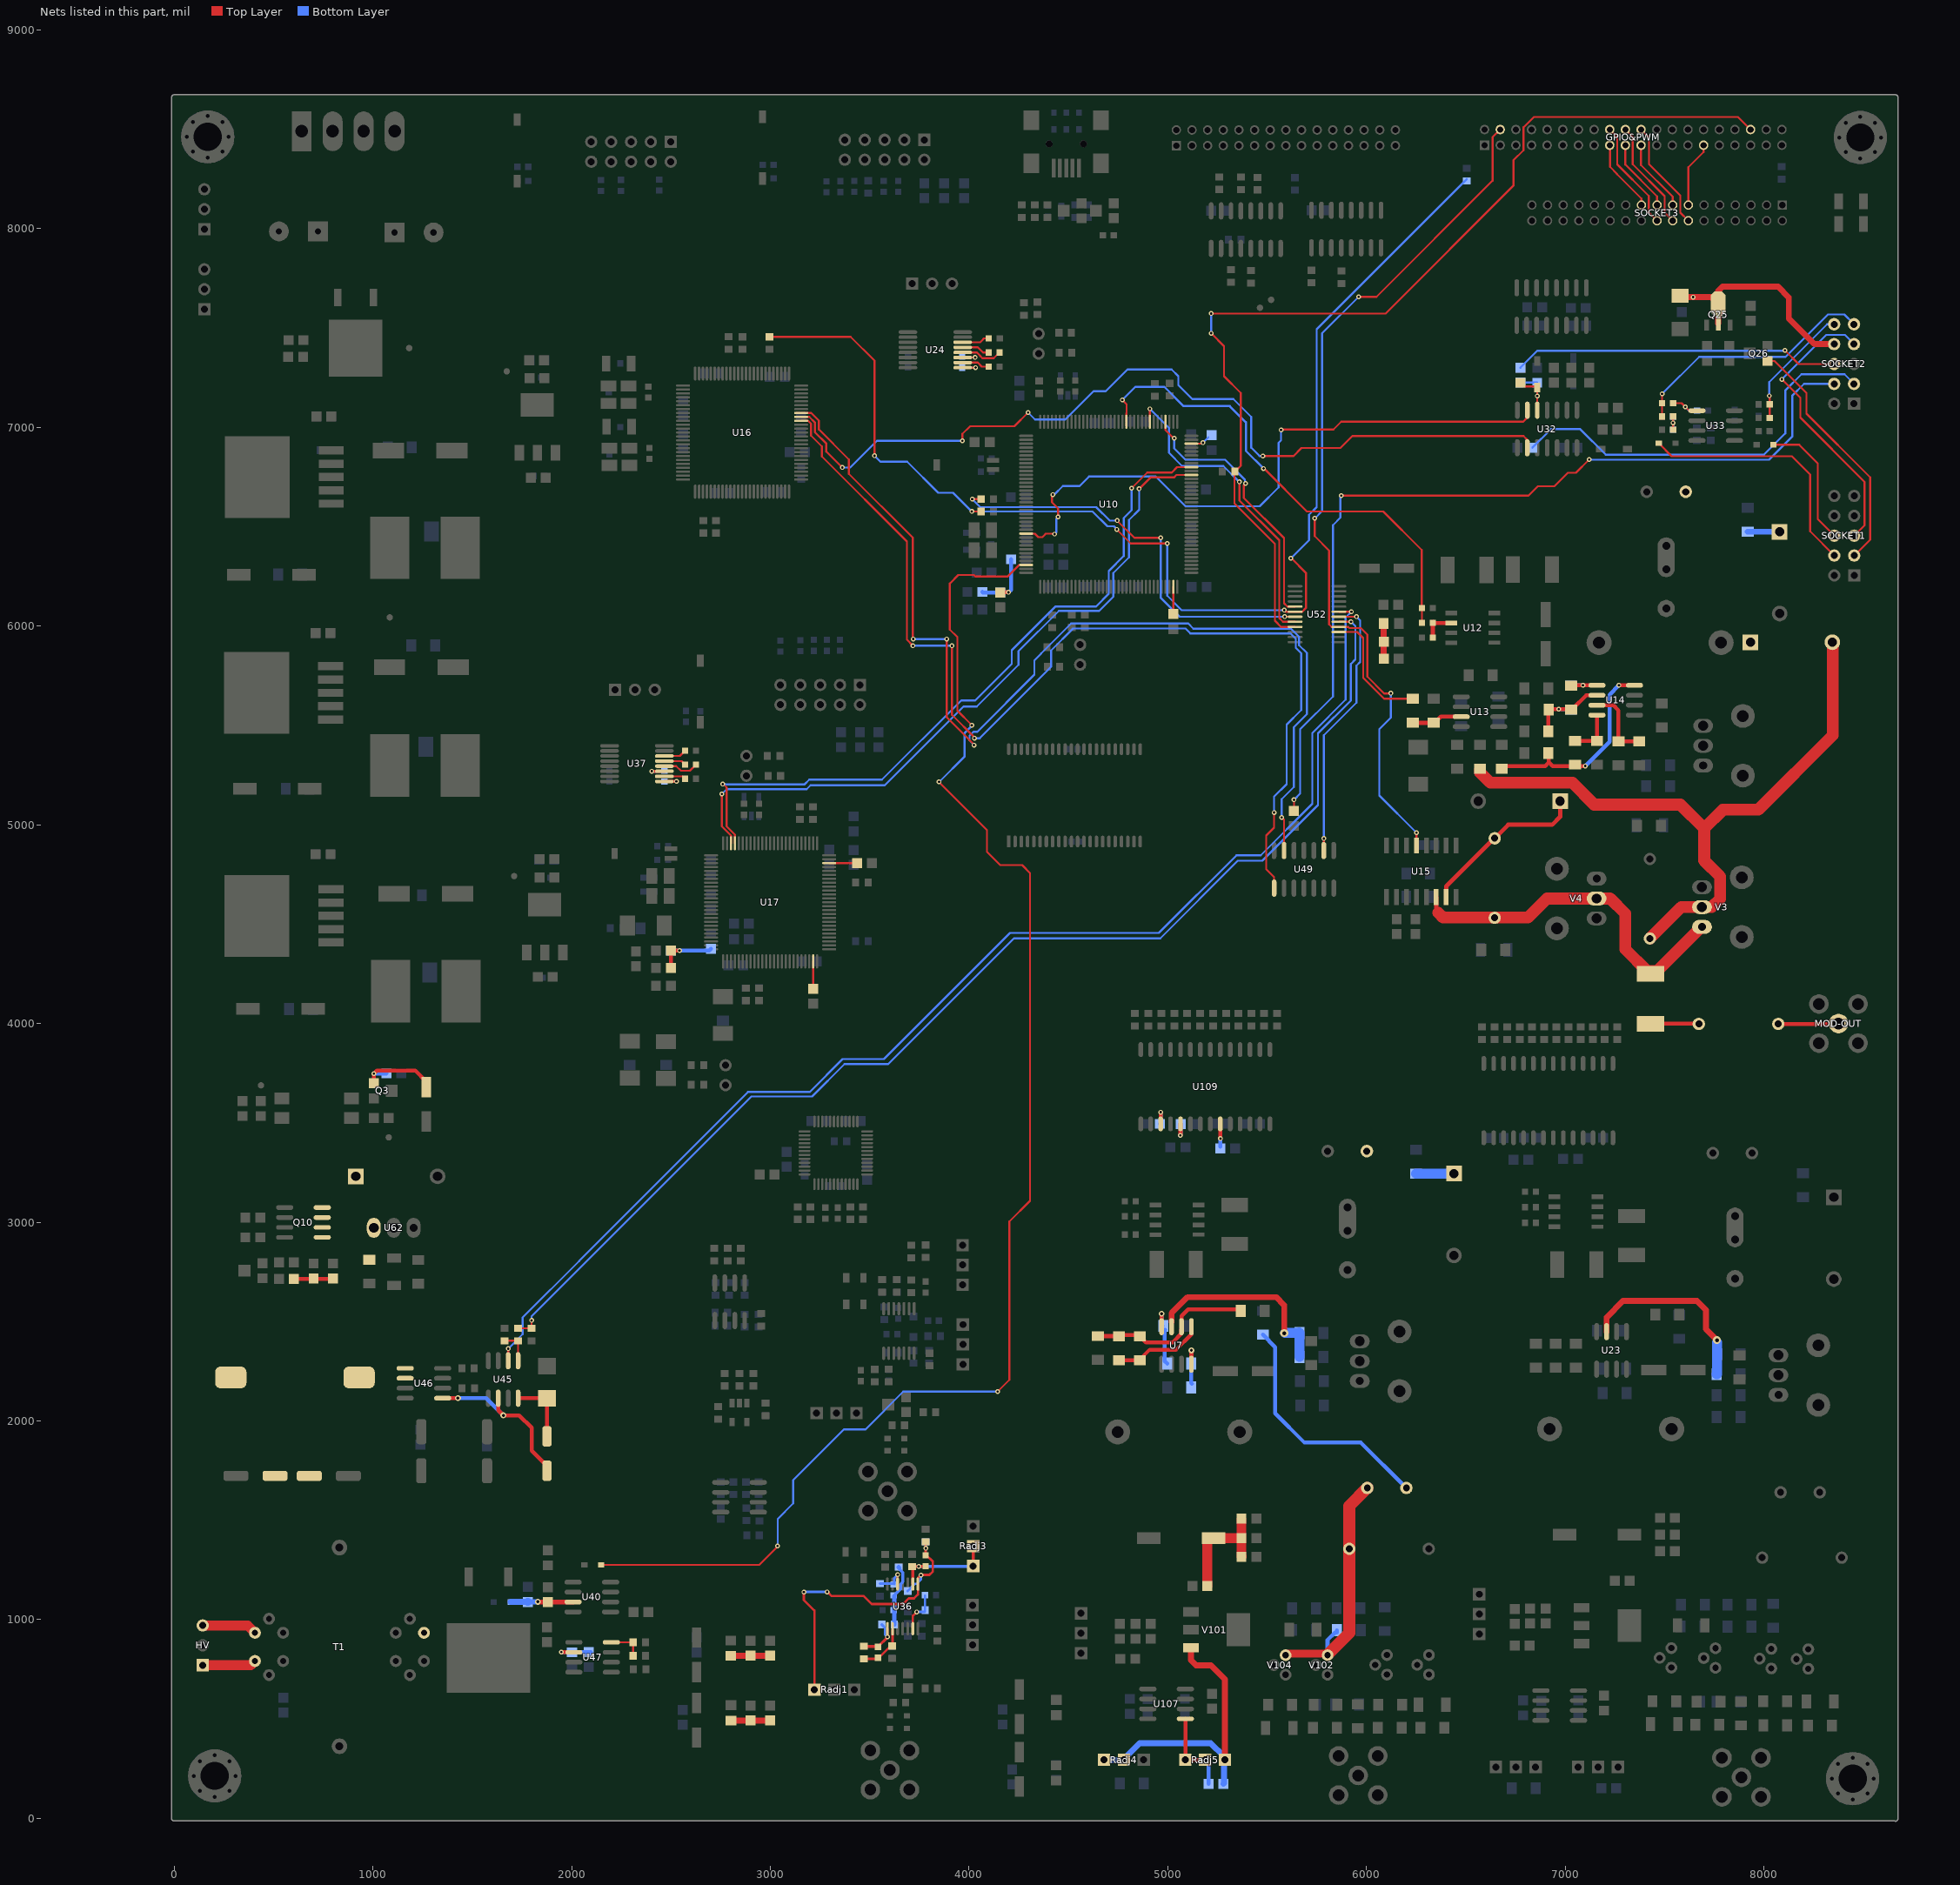
[diagram p0: the nets of this part, all layers, seen from the top]
# Altium PCB MISC82309.PcbDoc (part 9 of 14)
Units mil, origin at the board's own origin, x right, y up, seen from the top; angles counter-clockwise.
Board outline 8687.03 x 8687.86 mil, 4 copper layers (Top Layer, GND, POWER, Bottom Layer); 747 components, 583 nets, 2530 pads, 1834 vias.

## Via types
v1: diameter 24, hole 12, Top Layer to Bottom Layer, 1799 vias
v2: diameter 30, hole 15, Top Layer to Bottom Layer, 26 vias
v3: diameter 40, hole 20, Top Layer to Bottom Layer, 9 vias

## Nets (pads, with @x,y where several pads share a name; then routed paths per layer and width w, separated by ;. In a path a pad name is that pad's centre, name@x,y a point inside that pad or via, vN(x,y) a via of type N, cw(c..) or ccw(c..) an arc to the next point about the centre after c; other vN are vias at no path point) (continued)
HV-CLK: R347.2 R358.2 R391.2 U52.18 | length 6308.5
  Top Layer w10: R347.2@2996,7455.5 3404.5,7455.5 3524,7336 v1(3524,6857) ; v1(4014,6577) R391.2@4060.5,6577 ; v1(4744,6487) 4744,6486 4814,6416 v1(4997,6416) ; v1@5593.2,6072.8 U52.18@5640.76,6072.8 5676.8,6072.8 5695,6091 5695,6254 5695,6261 5695,6268 v1@5623,6340 ; v1@5619,6340 v1(5619,6342)
  Bottom Layer w10: v1(3524,6857) 3554,6827 3689,6827 3845,6671 3920,6671 v1(4014,6577) 4621,6577 4696,6502 4729,6502 v1(4744,6487) v1@4744,6486 ; v1(4997,6416) 4997,6153 5070,6080 v1(5586,6080) ; v1@5619,6340 v1(5619,6342) ; v1@5620,6342 5710.5,6432.5 5710.5,6560.5 5749,6599 5749,7494 R358.2@6504.5,8249.5
HV-CONTROL: U10.112 U52.17 | length 1331.3
  Top Layer w10: U10.112@4988.43,7028.35 4988.43,6986.57 5029,6946 v1(5032,6946) ; 5383,6709 5383,6645 5585,6443 5585,6115 5601.61,6098.39 U52.17@5640.76,6098.39
  Bottom Layer w10: v1(5032,6946) 5032,6894 5089,6837 5288,6837 5388,6737 5388,6731.06 5389,6730.06 v1@5389,6723 ; v1@5390,6719 v1(5391,6718)
HV-SHUTDOWN: U45.2 U52.7 | length 6403.5
  Top Layer w10: U45.2@1681,2303.49 v1(1681,2364) ; U52.7@5861.24,6072.8 v1(5924.2,6072.8)
  Bottom Layer w10: v1(1681,2364) 1754,2437 1754,2521 2038,2805 2038,2806 2888,3656 3199,3656 3364,3821 3571,3821 4206,4456 4955,4456 5346,4847 5468,4847 5727,5106 5727,5462 5895,5630 5895,6043.59 v1(5924.2,6072.8)
HV_CLK: U49.9 U52.6 | length 1352.7
  Top Layer w10: U49.9@5785,4870.49 v1(5785,4931) v1@5785,4937 ; U52.6@5861.24,6047.2 v1(5949.2,6047.2)
  Bottom Layer w10: v1(5785,4931) 5785,5451 5949.2,5615.2 5949.2,5801 5968,5819.8 5968,6029 v1@5953,6044 ; v1@5949.2,6044 v1(5949.2,6047.2)
HV_OUT+: HV.1 T1.7 | length 271.6
  Top Layer w50: HV.1@144,771 385.67,771 T1.7@406.8,792.13
HV_OUT-: HV.3 T1.8 | length 278.2
  Top Layer w50: HV.3@144,971 369.67,971 T1.8@406.8,933.87
HV_PWM: R285.1 R286.2 U52.5 | length 6220.6
  Top Layer w10: R285.1@1731,2466.5 R286.2@1799,2466.5 v1(1799,2506) ; U52.5@5861.24,6021.61 v1(5921.61,6021.61)
  Bottom Layer w10: v1(1799,2506) 1799,2527 2905,3633 3210,3633 3373,3796 3593,3796 4226,4429 4962,4429 5352,4819 5476,4819 5756,5099 5756,5460 5921.61,5625.61 5921.61,5810 5944.16,5832.54 5944.16,5999.84 v1@5923,6021 ; v1@5921.61,6021 v1(5921.61,6021.61)
HV_S: U10.26 U32.6 | length 3227.8
  Top Layer w10: U10.26@4287.65,6465.36 4330.7,6465.36 4348.06,6448 4369.06,6448 4379.03,6457.97 ; 4379,6458 4386,6465 4428,6465 v1(4430,6463) ; v1@4417,6657 4417,6623 4448,6592 v1(4448,6549) ; v1@5572,6989 5833,6989 5873,7029 6789,7029 6809,7049 U32.6@6809,7086.49
  Bottom Layer w10: v1(4422,6662) 4429,6662 4472,6705 4556,6705 4604,6753 4939,6753 5089,6603 5463,6603 5558,6698 5558,6769 ; 4439,6472 4439,6540 ; 5558,6775 5558,6769 ; 5558,6906 5558,6899 ; v1(5570,6987) 5570,6935 5558,6923 5558,6899 ; 5558,6769 5558,6899
HV_SENSOR: D33.2 U10.34 | length 7432.9
  Top Layer w10: D33.2@2149.32,1276 2944,1276 3038,1370 3037,1370 v1(3036,1371) ; v1@3848.5,5215.5 4090,4974 4090,4864 4157,4797 4267,4797 4307,4757 4307,3108 4203,3004 4203,2207 v1(4144,2148) ; v1@4012,5503 3941,5574 3941,5945 3903,5983 3903,6214 3946,6257 4025,6257 4033,6249 4193.6,6249 4252.48,6307.88 U10.34@4287.65,6307.88
  Bottom Layer w10: v1@3037,1370 3037,1507 3115,1585 3115,1703 3370,1958 3479,1958 3669,2148 v1(4144,2148) ; v1@3850,5217 3978,5345 3978,5463 v1@4013,5498
  other v1: 3849,5216 4014,5501
HV_SET: R392.2 U52.19 | length 2093.4
  Top Layer w10: v1(4016.17,6639.17) R392.2@4060.5,6639.17 ; v1(4746,6531) 4746,6530 4832,6444 v1(4964,6444) ; v1(5587.8,6047.2) U52.19@5640.76,6047.2
  Bottom Layer w10: v1(4016.17,6639.17) 4056.35,6599 4640,6599 4708,6531 v1@4744,6531 ; v1@4745,6530 v1@4744,6531 ; v1@4746,6530 v1(4746,6531) v1@4744,6531 ; v1(4964,6444) 4964,6143 5059.8,6047.2 v1(5587.8,6047.2)
HV_SINGLE: R166.1 SOCKET2.6 | length 1643.8
  Top Layer w10: v1(8105,7388) 8174,7319 SOCKET2.6@8353,7319
  Bottom Layer w10: R166.1@6774,7300.5 6859.05,7385.55 8077.45,7385.55 8102.55,7385.55 v1(8105,7388)
HV_VCC: C227.2 C228.2 L13.2 T1.2
INK-LED_A: R212.2 SOCKET2.3 | length 2023.2
  Bottom Layer w10: R212.2@6834.5,6898 6927.5,6991 7076,6991 7204,6863 8000,6863 8107,6970 8107,7185 8189,7267 8405,7267 SOCKET2.3@8453,7219
INK-LED_B: R386.2 SOCKET2.4 | length 4523.9
  Top Layer w10: R386.2@5635,5066 R386.2@5635,5069.5 v1(5635,5126) ; v1(5873,6657) 6815,6657 6862,6704 6945,6704 7013,6772 7054,6772 v1(7120,6838)
  Bottom Layer w10: v1(5635,5126) 5666,5157 5666,5481 5831,5646 5831,6508 5869,6546 5869,6653 v1(5873,6657) ; v1(7120,6838) 7121,6837 8026,6837 8142,6953 8142,7159 8202,7219 SOCKET2.4@8353,7219
INK_DETECTING: U10.98 U17.98 | length 3576.2
  Top Layer w10: v1@2757,5157 2756,5156 v1(2756,5155) 2756,4992 2802.15,4945.85 U17.98@2802.15,4907.24 ; v1(4856,6691) 4913,6748 5031,6748 5043.64,6760.64 U10.98@5118.35,6760.64
  Bottom Layer w10: v1@2758,5157 2780,5179 3183,5179 3203,5199 3576,5199 3972,5595 4039,5595 4249,5805 4249,5874 4452,6077 4655,6077 4726,6148 4726,6267 4805,6346 4805,6534 4856,6585 v1(4856,6691)
INK_FLOW_A: D31.2 SOCKET1.4 | length 1284.9
  Top Layer w10: D31.2@7470.68,6920 7535.68,6855 8140,6855 8232,6763 8232,6477 SOCKET1.4@8354,6355
INK_FLOW_B: D131.2 SOCKET1.6 | length 661
  Top Layer w10: D131.2@8047.32,6913 8177,6913 8271,6819 8271,6538 SOCKET1.6@8354,6455
INK_FLOW_SA: R172.2 R173.2 SOCKET2.9 | length 1264.8
  Top Layer w10: R173.2@7487.5,7055 R172.2@7487.5,7122 v1(7487.5,7168.5)
  Bottom Layer w10: v1(7487.5,7168.5) 7674,7355 8109,7355 8322,7568 8404,7568 SOCKET2.9@8453,7519
INK_FLOW_SB: R372.2 R373.2 SOCKET2.10 | length 625
  Top Layer w10: R373.2@8028.5,7048 R372.2@8028.5,7116 v1@8028.5,7157.5
  Bottom Layer w10: v1(8027,7159) 8027,7228 8318,7519 SOCKET2.10@8353,7519
INK_PRINTING: U10.100 U17.97 | length 3629.5
  Top Layer w10: v1@2762,5206 2780,5188 2780,4992.04 2821.83,4950.21 U17.97@2821.83,4907.24 ; v1(4818,6694) 4897.02,6773.02 5020.02,6773.02 5047,6800 U10.100@5118.35,6800.01
  Bottom Layer w10: v1@2765,5205 2766,5204 3173,5204 3196,5227 3562,5227 3961,5626 4031,5626 4215,5810 4215,5879 4434,6098 4638,6098 4703,6163 4703,6277 4779,6353 4779,6544 4818,6583 4818,6603 ; 4818,6596 4818,6603 ; v1(4818,6694) 4818,6603
  other v1: 2761,5205
INPUT0: GPIO&PWM.18 SOCKET3.18 | length 557.2
  Top Layer w10: GPIO&PWM.18@7223.92,8498.74 7254.83,8467.83 ; 7255,8468 7262,8461 7262,8323 7420,8165 7420,8082.34 SOCKET3.18@7462.08,8040.26
INPUT1: GPIO&PWM.19 SOCKET3.17 | length 367
  Top Layer w10: GPIO&PWM.19@7302.66,8420 7302.66,8322.34 7462.08,8162.92 SOCKET3.17@7462.08,8119
INPUT3: GPIO&PWM.17 SOCKET3.19 | length 371.6
  Top Layer w10: GPIO&PWM.17@7225,8425 7225,8311 7261,8275 7261,8274 7383.34,8151.66 SOCKET3.19@7383.34,8119
INPUT4: GPIO&PWM.21 SOCKET3.15 | length 367
  Top Layer w10: GPIO&PWM.21@7381.4,8420 7381.4,8320.6 7540.82,8161.18 SOCKET3.15@7540.82,8119
INPUT5: GPIO&PWM.20 SOCKET3.16 | length 557.1
  Top Layer w10: GPIO&PWM.20@7302.66,8498.74 7339,8462.4 7339,8325 7500,8164 7500,8081.08 SOCKET3.16@7540.82,8040.26
INPUT6: GPIO&PWM.29 SOCKET3.13 | length 332.8
  Top Layer w10: SOCKET3.13@7619.56,8119 7619.56,8309 7696.36,8385.8 GPIO&PWM.29@7696.36,8420
INPUT7: GPIO&PWM.22 SOCKET3.14 | length 557.1
  Top Layer w10: GPIO&PWM.22@7381.4,8498.74 7421,8459.14 7421,8325 7579,8167 7579,8080.82 SOCKET3.14@7619.56,8040.26
LASER_CTRL: Q26.1 SOCKET1.3 | length 1246.4
  Top Layer w10: Q26.1@8018,7334 8053,7334 8151,7236 8214,7173 8214,7069 8534,6749 8534,6435 SOCKET1.3@8454,6355
LASER_DRV: C221.2 D40.2 Q25.2 SOCKET2.8 | length 1205.2
  Top Layer w30: D40.2@7578,7662.86 7584.86,7656 7735.43,7656 Q25.2@7770,7621.43 ; Q25.2@7770,7523.01 Q25.2@7770,7621.43 ; SOCKET2.8@8353,7419 8254,7419 8125,7548 8125,7654 8071,7708 7791,7708 7770,7687 Q25.2@7770,7621.43
  Bottom Layer w30: C221.2@7585,7655.5 v1(7643.5,7655.5)
MCH_DRV: SOCKET1.5 SOCKET2.7 | length 1455.3
  Top Layer w10: v1(8090,7242) 8183,7149 8183,7049 8506,6726 8506,6507 SOCKET1.5@8454,6455
  Bottom Layer w10: v1(8090,7242) 8124.5,7276.5 8313,7465 8407,7465 SOCKET2.7@8453,7419
MOD-CLK: U16.66 U49.1 | length 5363.3
  Top Layer w10: U16.66@3155.24,7033.06 3190.41,7033.06 3205,7018.46 3205,6959 3259.83,6904.17 3259.83,6853.17 3687,6426 3687,5932 v1(3718,5901) ; v1(3914,5901) 3914,5554 4029,5439 v1@4029,5438 ; 5534,4738 5495,4777 5495,4946 5535,4986 v1(5535,5062) ; U49.1@5535,4681.51 5535,4738
  Bottom Layer w10: v1(3718,5901) v1(3914,5901) ; v1(4027,5436) 4054,5436 4413,5795 4413,5877 4524,5988 5089,5988 5114,5963 5618,5963 5644,5937 5644,5891 5671.5,5863.5 5671.5,5577.5 5598,5504 5598,5205 5535,5142 v1(5535,5062)
MOD-CONTROL: U10.116 U52.20 | length 1597.8
  Top Layer w10: U10.116@4909.69,7028.35 v1(4909.69,7093.31) ; v1@5361,6727 5361,6632 5561,6432 5561,6040.06 5579.44,6021.61 U52.20@5640.76,6021.61
  Bottom Layer w10: v1(4909.69,7093.31) 5006,6997 5006,6872 5072,6806 5280,6806 v1(5360,6726)
MOD-LED_A: U16.67 U32.9 | length 4451.5
  Top Layer w10: U16.67@3155.24,7052.74 3196.26,7052.74 3224,7025 3224,6976 3282,6918 3282,6878 v1(3362,6798) ; v1(3967,6933) 3967,6967 4006,7006 4228,7006 v1(4297,7075) ; v1(5478,6856) 5633,6856 5673,6896 5868,6896 5929,6957 6790,6957 6809,6938 U32.9@6809,6897.51
  Bottom Layer w10: v1(3362,6798) 3402,6798 3537,6933 v1(3967,6933) ; v1(4297,7075) 4332,7040 4484,7040 4626,7182 4688,7182 4797,7291 5019,7291 5053,7257 5053,7213 5123,7143 5330,7143 5420,7053 5420,6898 5462,6856 v1(5478,6856)
MOD-LED_B: U16.68 U49.13 | length 5310.6
  Top Layer w10: U16.68@3155.24,7072.43 3205.57,7072.43 3244.07,7033.93 3244.07,6989.93 3395.47,6838.53 3395.47,6766.53 3717,6445 v1@3717,5937 ; v1(3888,5935) 3888,5542 4003,5427 ; 4003,5426.06 4017.06,5412 ; v1(5573,5037) 5585,5025 U49.13@5585,4870.49
  Bottom Layer w10: v1(3719,5935) v1(3888,5935) ; v1@4024,5403 4003,5424 4003,5449 4022.5,5468.5 4041.5,5468.5 4329,5756 4329,5827 4363,5861 ; v1(4025,5401) v1@4025,5405 ; 4363,5862 4514,6013 5103,6013 5129,5987 5620,5987 5661,5946 5661,5904 5700,5865 5700,5557 5634,5491 5634,5190 5573,5129 v1(5573,5037)
MOD-PWM: R72.2 U52.3 | length 626.9
  Top Layer w10: U52.3@5861.24,5970.43 5952.57,5970.43 5983,5940 5983,5740 6088,5635 R72.2@6232,5635
MOD-SET: GPIO&PWM.36 R508.2 U52.21 | length 5112
  Top Layer w10: v1(5218,7474) 5283,7409 5283,7257 5367,7173 5367,6807 5336,6776 5336,6617 5539,6414 5539,6027 5569.98,5996.02 U52.21@5640.76,5996.02 ; v1(5218,7573) 6096,7573 6739,8216 6739,8344 6790,8395 6790,8510 6842,8562 7869.32,8562 GPIO&PWM.36@7932.58,8498.74
  Bottom Layer w10: v1(5218,7474) v1(5218,7573)
MOD-SHUTDOWN: GPIO&PWM.4 U15.13 U52.4 | length 4403.1
  Top Layer w10: v1@5738,6543 v1(5739,6543) ; v1@5739,6542 5739,6453 5811.83,6380.17 5811.83,6009.17 U52.4@5824.98,5996.02 ; U52.4@5829.02,5996.02 U52.4@5861.24,5996.02 5907.98,5996.02 5914,5990 5971,5990 6004,5957 6004,5746 6089,5661 6123,5661 v1(6122,5662) ; v1(5960,7657) 6050,7657 6634,8241 6634,8460 GPIO&PWM.4@6672.74,8498.74 ; U15.13@6251,4896 v1(6251,4960)
  Bottom Layer w10: v1@5738,6541 5739,6541 5776,6578 5776,7473 v1(5960,7657) ; v1@6122,5659 6122,5539 6064,5481 6064,5147 v1(6251,4960)
MOD_CTRL: R67.2 R68.2 U10.122 | length 2439.6
  Top Layer w10: v1(4771,7138) 4793,7116 4793,7073 4791.58,7071.58 U10.122@4791.58,7028.35 ; v1(5482,6793) 5484,6793 5700,6577 6084,6577 6278,6383 R68.2@6278,6095 ; R67.2@6278.5,6016 R68.2@6278.5,6089.5
  Bottom Layer w10: v1(4771,7138) 4837,7204 4983,7204 5080,7107 5312,7107 5393,7026 5393,6882 v1(5482,6793)
MOD_OUT: C62.2 MOD-OUT.1 | length 286.8
  Top Layer w20: C62.2@8072,3998 8356,3998 MOD-OUT.1@8358,3996
NetC17_2: C17.2 Q3.1 R15.1 | length 427.9
  Top Layer w20: Q3.1@1005,3699 v1(1005,3748) ; v1@1007,3749 1021,3763 1214,3763 1268,3709 C17.2@1268,3692 ; C17.2@1269,3680.23 C17.2@1269,3692
  Bottom Layer w20: v1@1008,3748 1067.5,3748 R15.1@1068.5,3749
NetC23_1: C23.1 R17.2 R18.1 R38.2 U7.2 | length 851.8
  Top Layer w15: R38.2@4848,2427 R38.2@4852,2423 ; R38.2@4860,2426 R38.2@4860,2432
  Top Layer w20: R17.2@4648,2427 4751,2427 4756,2432 4860,2432 R38.2@4861,2431 ; R38.2@4860,2426 4890,2396 5025,2396 5068,2439 U7.2@5068,2461 ; U7.2@5069,2474.49 5069,2529 5102,2562 5361,2562 R18.1@5364,2559
NetC23_2: C23.2 R38.1 U7.1 | length 450.3
  Top Layer w20: C23.2@4755,2306 4856,2306 4909,2359 5042,2359 5120,2437 U7.1@5120,2468
NetC24_1: C24.1 R26.1 U7.8 | length 256.1
  Top Layer w20: U7.8@5119,2268 U7.8@5119,2285.51 v2(5119,2355)
  Bottom Layer w20: v2@5118,2355 5117,2354 R26.1@5117,2289 5117,2192 C24.1@5121,2188
NetC25_1: C25.1 R26.2 U7.4 | length 303.6
  Top Layer w20: U7.4@4969,2474.49 v2(4969,2540)
  Bottom Layer w20: v2(4969,2540) 4969,2483 C25.1@4973,2479 ; C25.1@4986,2459 4985,2458 4985,2301 R26.2@4997,2289
NetC27_1: C27.1 R25.1 U7.3 | length 1025.5
  Top Layer w20: U7.3@5019,2474.49 U7.3@5019,2499
  Top Layer w30: U7.3@5019,2499 5019,2542 5100,2623 5545,2623 5586,2582 v3(5586,2442)
  Bottom Layer w20: v3@5586,2443 5587,2442 v3@5591,2442
  Bottom Layer w50: v3@5591,2444 5658,2444 5660,2446 5663,2443 C27.1@5663,2442 R25.1@5663,2322
NetC29_1: C29.1 D5.2 L111.1 R19.2 R39.2 | length 1413.4
  Bottom Layer w20: R19.2@5479,2434 5541,2372 5541,2038 5688,1891 5972,1891 L111.1@6192,1671
  Bottom Layer w50: R39.2@6249,3245 6432,3245 D5.2@6436,3241
NetC30_2: C30.2 U109.19 | length 117.4
  Top Layer w20: v1(5063,3437) 5064,3438 U109.19@5064,3494.99
  Bottom Layer w20: v1@5062,3436 v1(5063,3437) 5064.5,3438.5 C30.2@5064.5,3494
NetC32_1: C32.1 U109.17 | length 119.5
  Top Layer w20: U109.17@4964,3494.99 v1(4964,3554)
  Bottom Layer w20: C32.1@4960.5,3495 4964,3498.49 v1(4964,3554)
NetC33_2: C33.2 U109.23 | length 115.8
  Top Layer w20: U109.23@5264,3494.99 5264,3422 v1(5265,3421)
  Bottom Layer w20: C33.2@5264,3380 5265,3381 v1(5265,3421)
NetC35_2: C35.2 C36.2 L11.2 R276.1 | length 326.3
  Top Layer w20: C36.2@4157,6168.5 4158.51,6170 v1(4199,6170)
  Bottom Layer w20: L11.2@4066.5,6172 4070,6168.5 C35.2@4143,6168.5 ; C35.2@4157,6168.5 4158.5,6170 v1@4198,6170 ; v1@4204,6175 4211.5,6182.5 R276.1@4211.5,6336
NetC42_2: C42.2 R67.1 U12.2 | length 174.1
  Top Layer w20: R67.1@6331,6013.5 R67.1@6333.5,6016 C42.2@6333.5,5940.5 ; R67.1@6334,6021 6339,6016 U12.2@6427,6016
NetC45_1: C45.1 R72.1 U13.3 | length 255.4
  Top Layer w20: R72.1@6234,5513 6343,5513 6374,5544 U13.3@6476.51,5544
NetC47_1: C47.1 R77.2 U14.1 | length 165.9
  Top Layer w20: C47.1@7043,5702 v1(7089,5702) 7091,5702 U14.1@7159.51,5702
  Bottom Layer w20: R77.2@7040,5703 7041,5702 v1(7089,5702)
NetC47_2: C47.2 R76.2 R77.1 R78.2 U14.2 | length 431.3
  Top Layer w20: R76.2@6915,5470 6915,5580 6917,5582 v1(6967,5582) 7028,5582 C47.2@7030,5580 ; C47.2@7035,5584 7038,5584 7106,5652 U14.2@7159.51,5652
  Bottom Layer w20: v1(6967,5582) R77.1@7019,5582
NetC48_1: C48.1 R75.2 U14.4 | length 234.8
  Top Layer w20: R75.2@7049,5423 7158,5423 7160,5425 U14.4@7160,5548
NetC49_1: C49.1 R73.1 R75.1 U14.8 | length 1037.3
  Top Layer w20: R73.1@6681,5283 6694,5296 6899,5296 6916,5313 6916,5358 C49.1@6915,5359 ; 6916,5317 6937,5296 7036,5296 7037,5297 R75.1@7045,5297 ; R75.1@7049,5303 7056,5296 v1(7101,5296) ; v1@7274,5702 U14.8@7348.49,5702
  Bottom Layer w20: v1(7101,5296) 7223,5418 7223,5655 v1(7270,5702)
NetC51_1: C51.1 R82.1 U14.3 | length 367.2
  Top Layer w20: U14.3@7166,5601 7243,5601 7268,5576 C51.1@7268,5420 R82.1@7364,5420 ; R82.1@7370,5422 R82.1@7372,5420
NetC54_1: C54.1 D11.2 D13.2 R74.2 | length 142
  Bottom Layer w30: R74.2@7918,6475 D13.2@8060,6475
NetC55_2: C55.2 D11.1 R71.1 V3.2 | length 3387.1
  Top Layer w60: R71.1@6571,5262 R71.1@6571,5276 ; R71.1@6571,5277 R71.1@6571,5276 ; C55.2@7427,4429 7584,4586 V3.2@7688,4586 7737,4586 7779,4628 7779,4740 7699,4820 7699,4982 ; D11.1@8347,5903 8346,5902 8346,5451 7971,5076 7793,5076 7699,4982 ; R71.1@6571,5276 6571,5264 6623,5212 7036,5212 7146,5102 7579,5102 7699,4982
NetC58_1: C58.1 R89.1 U15.6 V3.3 V4.2 | length 1801.7
  Top Layer w20: U15.6@6351,4636 6351,4582 6368,4565
  Top Layer w60: 6361,4558 6386,4533 6812,4533 6908,4629 V4.2@7158,4629 7226,4629 7302,4553 7302,4374 7412,4264 7462,4264 7683,4485 V3.3@7687,4485
NetC58_2: C58.2 D15.2 U15.7 | length 837.6
  Top Layer w22: U15.7@6401,4636 6401,4690 C58.2@6636,4925 ; C58.2@6634.5,4926.5 C58.2@6637,4929 ; C58.2@6645,4932 6713,5000 6934,5000 6974,5040 D15.2@6974,5114
NetC62_1: C62.1 R89.2 | length 235.4
  Top Layer w20: R89.2@7430,3999.02 C62.1@7663.98,3999.02
  Top Layer w30: C62.1@7663.98,3999.02 C62.1@7665,3998
NetC66_2: C66.2 FB3.2 R91.1 | length 175.9
  Top Layer w30: FB3.2@6082,6010 6086.5,6005.5 C66.2@6086.5,5921 6086.5,5920.5 R91.1@6086.5,5836
NetC70_2: C70.2 C71.2 L14.2 R225.1 | length 336.9
  Top Layer w20: L14.2@2499.5,4280 C70.2@2499.5,4367 v1(2542.99,4366.99)
  Bottom Layer w20: C71.2@2499.5,4367 2559,4367 2692.5,4367 R225.1@2702,4376.5
NetC78_1: C78.1 D10.2 Q10.5 Q10.6 Q10.7 Q10.8 U62.1
NetC91_1: C91.1 U24.3 | length 129.8
  Top Layer w10: U24.3@3967.8,7351.61 4030.61,7351.61 v1(4031,7352)
  Bottom Layer w10: C91.1@3966,7355.5 3969.5,7352 v1(4031,7352)
NetC91_2: C91.2 U24.1 | length 132.6
  Top Layer w10: U24.1@3967.8,7300.43 4032.43,7300.43 v1(4033,7301)
  Bottom Layer w10: C91.2@3966,7300.5 4032.5,7300.5 v1(4033,7301)
NetC92_1: C92.1 U24.5 | length 141.4
  Top Layer w10: U24.5@3967.8,7402.8 4044.2,7402.8 4070,7377 C92.1@4098.5,7377
NetC92_2: C92.2 U24.4 | length 211
  Top Layer w10: U24.4@3967.8,7377.2 4039.74,7377.2 4055,7361.94 4055,7360 4067,7348 4124.5,7348 C92.2@4153.5,7377
NetC93_2: C93.2 U24.2 | length 139
  Top Layer w10: U24.2@3967.8,7326.02 4043.98,7326.02 4064,7306 C93.2@4098.5,7306
NetC94_2: C94.2 U24.6 | length 140.4
  Top Layer w10: U24.6@3967.8,7428.39 4056.33,7428.39 4072,7444.06 4072,7445 4075,7448 C94.2@4099.5,7448
NetC157_1: C157.1 R44.2 R45.2 R46.1 TC2.2 | length 564.2
  Top Layer w50: R44.2@5199.5,1170 5199.5,1400.5 TC2.2@5205,1406 ; TC2.2@5230.77,1411 R46.1@5370,1411 ; R45.2@5370.5,1505.5 R46.1@5370.5,1411 5370.5,1319.5 C157.1@5371,1319
NetC162_2: C162.2 D24.2 R166.2 R168.2 U32.5 | length 360.6
  Top Layer w10: C162.2@6774,7224.5 6792.5,7206 6853.07,7206 D24.2@6859,7200.07 U32.5@6859,7086.49
  Bottom Layer w10: R166.2@6774,7225.5 6858,7225.5 R168.2@6859,7224.5 v1(6859,7158)
NetC163_1: C163.1 R173.1 R174.1 R175.2 | length 134.5
  Top Layer w10: R175.2@7542.5,6988 R173.1@7542.5,7055
  Bottom Layer w10: v1(7542,7023) v1@7542.5,7023 ; C163.1@7542.5,6988 v1@7542.5,7023 ; R174.1@7542.5,7055 v1@7542.5,7023
NetC164_2: C164.2 R172.1 U33.5 | length 203.1
  Top Layer w10: R172.1@7542.5,7122 7586,7122 7624,7084 U33.5@7662.51,7084
  Bottom Layer w10: v1(7604,7103) 7623,7084 C164.2@7663.5,7084
NetC166_1: C166.1 R187.2 R188.1 U36.1 | length 245.2
  Top Layer w14: R187.2@3480,865 3543,865 3589.23,911.23 U36.1@3589.23,954.8
  Bottom Layer w14: R188.1@3561.5,975 R188.1@3564.25,972.25 ; R188.1@3564,972 3578,958 3578,924 v1(3589,913)
NetC166_2: C166.2 R186.2 R187.1 U36.2 | length 248
  Top Layer w12: R187.1@3470,803.5 3541.5,803.5 3609,871 3610,871 3615,876 U36.2@3615,949
NetC167_1: C167.1 C168.2 R188.2 R189.1 | length 304.1
  Bottom Layer w15: C168.2@3630,1129 3655,1154 3655,1179 ; R189.1@3651,1262 3651,1253.48 3667.5,1236.98 3667.5,1225 3667.5,1215.02 3667.5,1190.5 3656,1179
  Bottom Layer w20: C168.2@3623,1120 3624,1119 3624,975.5 R188.2@3624.5,975 ; R189.1@3646,1262.01 R189.1@3646,1265.5
NetC168_1: C168.1 R192.2 U36.12 | length 167
  Top Layer w12: U36.12@3640.41,1179.2 3640.41,1225.41 v1(3641,1226)
  Bottom Layer w12: R192.2@3552,1181.5 3621.5,1181.5 3624,1179 3624,1209 v1@3636,1221
NetC169_1: C169.1 D27.1 R195.2 R196.2 Radj1.3 U36.8 | length 1614.2
  Top Layer w12: v1(3169,1139) 3169,1099 3222,1046 Radj1.3@3222,648 ; v1@3288,1140 3309,1119 3470,1119 3510,1079 3669,1079 3697,1107 3723,1107 3742.77,1126.77 U36.8@3742.77,1179.2 3742.77,1210.77 3757,1225 3800,1225 3818,1243 3818,1292 3782,1328 R196.2@3782,1392
  Bottom Layer w12: v1(3169,1139) 3170,1140 v1(3286,1140) ; D27.1@3691,1144 3728,1181 3738,1181 3758,1201 v1(3758,1224) ; R195.2@3782,1392.5 3782,1360 v1(3783,1359)
NetC169_2: C169.2 R194.2 Radj3.2 Radj3.3 U36.9 | length 495.2
  Top Layer w14: U36.9@3717.18,1179.2 R194.2@3717.18,1254.82 ; R194.2@3717.18,1261.82 3717,1262 3723,1268 v1(3747,1268) C169.2@3777,1268 ; Radj3.3@4021,1277 4021,1366 Radj3.2@4023,1368
  Bottom Layer w14: v1(3747,1268) 3846,1268 Radj3.3@4012,1268
NetC170_1: C170.1 R200.1 U36.6 | length 214.2
  Top Layer w12: U36.6@3717.18,954.8 3717.18,1019.18 v1(3737,1039)
  Bottom Layer w12: v1(3737,1039) 3776,1039 3778,1041 C170.1@3778,1121
NetC173_2: C173.2 FB19.2 R204.1 | length 198.4
  Top Layer w30: FB19.2@2802,492.61 R204.1@3000.39,492.61
NetC176_2: C176.2 FB20.2 R205.1 | length 189.4
  Top Layer w30: FB20.2@2801,818.61 R205.1@2990.39,818.61
NetC177_1: C177.1 U37.3 | length 124.8
  Top Layer w15: v1(2403.61,5269.61) U37.3@2466.8,5269.61
  Bottom Layer w15: v1(2403.61,5269.61) 2404.23,5269 C177.1@2465,5269
NetC177_2: C177.2 U37.1 | length 117.3
  Top Layer w15: U37.1@2466.8,5218.43 v1(2527.57,5218.43)
  Bottom Layer w15: C177.2@2467,5217.5 v1@2523.5,5217.5
NetC178_1: C178.1 U37.5 | length 112.1
  Top Layer w10: U37.5@2466.8,5320.8 2553.7,5320.8 C178.1@2571.5,5303
NetC178_2: C178.2 U37.4 | length 182.2
  Top Layer w10: U37.4@2466.8,5295.2 2526.8,5295.2 2550,5272 2595.5,5272 C178.2@2626.5,5303
NetC179_2: C179.2 U37.2 | length 109.7
  Top Layer w10: U37.2@2466.8,5244.02 2559.48,5244.02 C179.2@2571.5,5232
NetC180_2: C180.2 U37.6 | length 115.7
  Top Layer w10: U37.6@2466.8,5346.39 2544.89,5346.39 C180.2@2571.5,5373
NetC184_2: C184.2 D32.2 R216.2 U40.3 | length 316.1
  Top Layer w25: v2(1830,1090) 1831.5,1088.5 R216.2@1881,1088.5 1881.5,1089 U40.3@2007.51,1089
  Bottom Layer w20: v2@1829.5,1089.5 v2(1830,1090)
  Bottom Layer w25: C184.2@1780.5,1090 v2(1830,1090)
  Bottom Layer w30: D32.2@1693.32,1089 C184.2@1779.5,1089
  Bottom Layer w40: C184.2@1779.5,1089 C184.2@1780,1089.5 C184.2@1780.5,1090
NetC187_1: C187.1 Radj4.1 Radj4.2 Radj5.3 V101.3 | length 1466.6
  Top Layer w30: V101.3@5116,858.45 5116,796 5142,770 5218,770 5288,700 Radj5.3@5288,299
  Bottom Layer w30: Radj4.1@4694,294 4774,294 4859,379 5216,379 5283,312 5283,177.49 C187.1@5279.5,174
NetC187_2: C187.2 Radj5.1 Radj5.2 U107.1 | length 437.7
  Top Layer w20: Radj5.1@5088,295 Radj5.2@5188,295 5190,295 Radj5.2@5193,292 ; U107.1@5088.49,501 5088.49,305.51 Radj5.1@5089,305
  Bottom Layer w20: C187.2@5204.5,174 5204.5,308.5 Radj5.2@5205,309
NetC188_2: C188.2 L111.2 R153.2 V102.3 V104.3 | length 1281.2
  Top Layer w20: V102.3@5795.79,821.21 V102.3@5798,819
  Top Layer w40: V104.3@5593,821.21 5600.32,828.53 5805.47,828.53 5807.5,826.5 V102.3@5808,826
  Top Layer w50: V102.3@5807.5,826.5 V102.3@5808.5,827.5
  Top Layer w60: V102.3@5808,828 5913,933 C188.2@5913,1357 5913,1572.43 L111.2@6003.57,1663
  Bottom Layer w20: V102.3@5804,821.21 5804,898 R153.2@5842,936 ; R153.2@5851,936 R153.2@5851,947
NetC193_2: C193.2 R8.2 R12.1 | length 197.9
  Top Layer w20: R12.1@602.5,2714 795.5,2714 R8.2@799,2717.5
NetC214_1: C214.1 U10.106 | length 98.9
  Top Layer w10: U10.106@5118.35,6918.12 5172.12,6918.12 v1(5177,6923)
  Bottom Layer w10: v1(5177,6923) C214.1@5204,6950
NetC215_1: C215.1 U10.71 | length 137.2
  Top Layer w10: U10.71@5027.8,6197.65 5028,6197.45 C215.1@5028,6060.5
NetC226_2: C226.2 R285.2 U45.1 | length 169
  Top Layer w10: C226.2@1662,2403.5 R285.2@1731,2403.5 U45.1@1731,2303.49
NetC229_1: C229.1 L13.1 U45.6 U46.1 U46.5 U46.6 | length 855
  Top Layer w20: U46.1@1351.49,2115 v2(1428,2115) ; U45.6@1631,2114.51 1631,2054 v2(1657,2028) 1737,2028 1799,1966 1799,1850 1876,1773 C229.1@1876,1749.39
  Bottom Layer w20: v2(1428,2115) 1570,2115 v2(1657,2028)
NetC229_2: C229.2 D38.2 U45.8 | length 336.5
  Top Layer w20: U45.8@1731,2114.51 1875.39,2114.51 D38.2@1876,2113.9 C229.2@1876,1922.61
NetC232_2: C232.2 R288.2 U47.4 | length 177
  Top Layer w10: U47.4@2200.49,886 C232.2@2309.5,886 R288.2@2309.5,818
NetC233_2: C233.2 FB27.1 U47.6 | length 213.2
  Top Layer w20: v1(1948,837) 1949,836 U47.6@2011.51,836
  Bottom Layer w20: v1(1948,837) 1948.61,836.39 2012,836.39 2096.89,836.39 C233.2@2097,836.5
NetC256_1: C256.1 U17.49 | length 137.4
  Top Layer w10: U17.49@3215.54,4312.76 3215.54,4175.96 C256.1@3216,4175.5
NetC257_1: C257.1 U17.73 | length 140.3
  Top Layer w10: U17.73@3296.24,4806.85 3436.35,4806.85 C257.1@3436.5,4807
NetC263_1: C263.1 R159.1 U23.3 | length 965.3
  Top Layer w30: U23.3@7208,2449.49 7208,2522 7290,2604 7663,2604 7708,2559 7708,2463 v3@7763.5,2407.5
  Bottom Layer w30: C263.1@7760,2324 C263.1@7763,2321
  Bottom Layer w50: R159.1@7762,2235 7763,2236 7763,2321 C263.1@7763,2336 v3@7763,2396
  other v3: 7763,2407